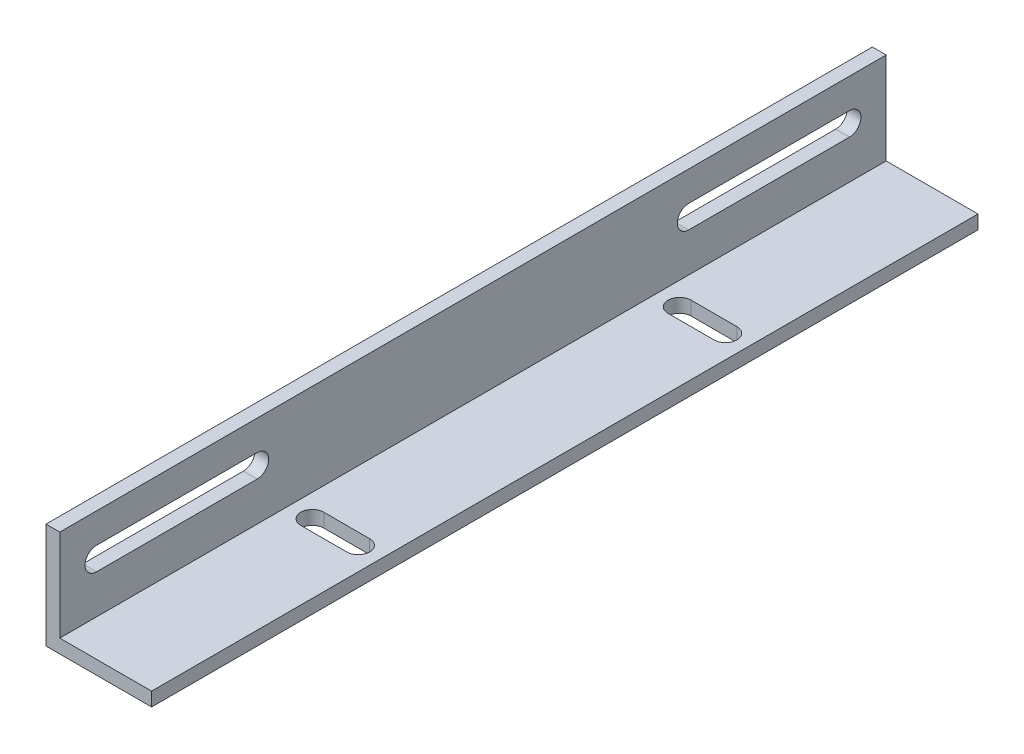
from build123d import *

# Parameters (mm, degrees)
EXTRUDE_1_DEPTH     = 90
CUT_EXTRUDE_1_REACH = 97.021
CUT_EXTRUDE_2_REACH = 97.021


with BuildPart() as part:
    # 草图1 → 凸台-拉伸1 (new, symmetric)
    with BuildSketch(Plane.XY):
        Polygon((0, 0), (0, 23), (3, 23), (3, 3), (23, 3), (23, 0), align=None)
    extrude(amount=EXTRUDE_1_DEPTH, both=True)

    # 草图3 → 切除-拉伸1 (cut, up to next)
    with BuildSketch(Plane(origin=(3, 0, 0), x_dir=(0, 0, -1), z_dir=(1, 0, 0)), mode=Mode.PRIVATE) as cut_extrude_1_sk1:
        with BuildLine():
            Line((-82, 16.5), (-47, 16.5))
            ThreePointArc((-47, 16.5), (-44.5, 14), (-47, 11.5))
            Line((-47, 11.5), (-82, 11.5))
            ThreePointArc((-82, 11.5), (-84.5, 14), (-82, 16.5))
        make_face()
    cut_extrude_1_tool1 = extrude(cut_extrude_1_sk1.sketch, amount=-CUT_EXTRUDE_1_REACH, mode=Mode.PRIVATE) & part.part
    cut_extrude_1 = cut_extrude_1_tool1.solids().sort_by_distance((3, 14, 64.5))[0]
    add(cut_extrude_1, mode=Mode.SUBTRACT)

    # 镜向1: 切除-拉伸1 across plane
    add(cut_extrude_1.mirror(Plane.XY), mode=Mode.SUBTRACT)

    # 草图4 → 切除-拉伸2 (cut, up to next)
    with BuildSketch(Plane(origin=(0, 3, 0), x_dir=(1, 0, 0), z_dir=(0, 1, 0)), mode=Mode.PRIVATE) as cut_extrude_2_sk1:
        with BuildLine():
            Line((8, 42.5), (18, 42.5))
            ThreePointArc((18, 42.5), (20.5, 40), (18, 37.5))
            Line((18, 37.5), (8, 37.5))
            ThreePointArc((8, 37.5), (5.5, 40), (8, 42.5))
        make_face()
    cut_extrude_2_tool1 = extrude(cut_extrude_2_sk1.sketch, amount=-CUT_EXTRUDE_2_REACH, mode=Mode.PRIVATE) & part.part
    # 草图4 → 切除-拉伸2 (cut, up to next)
    with BuildSketch(Plane(origin=(0, 3, 0), x_dir=(1, 0, 0), z_dir=(0, 1, 0)), mode=Mode.PRIVATE) as cut_extrude_2_sk2:
        with BuildLine():
            Line((8, -37.5), (18, -37.5))
            ThreePointArc((18, -37.5), (20.5, -40), (18, -42.5))
            Line((18, -42.5), (8, -42.5))
            ThreePointArc((8, -42.5), (5.5, -40), (8, -37.5))
        make_face()
    cut_extrude_2_tool2 = extrude(cut_extrude_2_sk2.sketch, amount=-CUT_EXTRUDE_2_REACH, mode=Mode.PRIVATE) & part.part
    add(cut_extrude_2_tool1.solids().sort_by_distance((13, 3, -40))[0], mode=Mode.SUBTRACT)
    add(cut_extrude_2_tool2.solids().sort_by_distance((13, 3, 40))[0], mode=Mode.SUBTRACT)


solid = part.part
